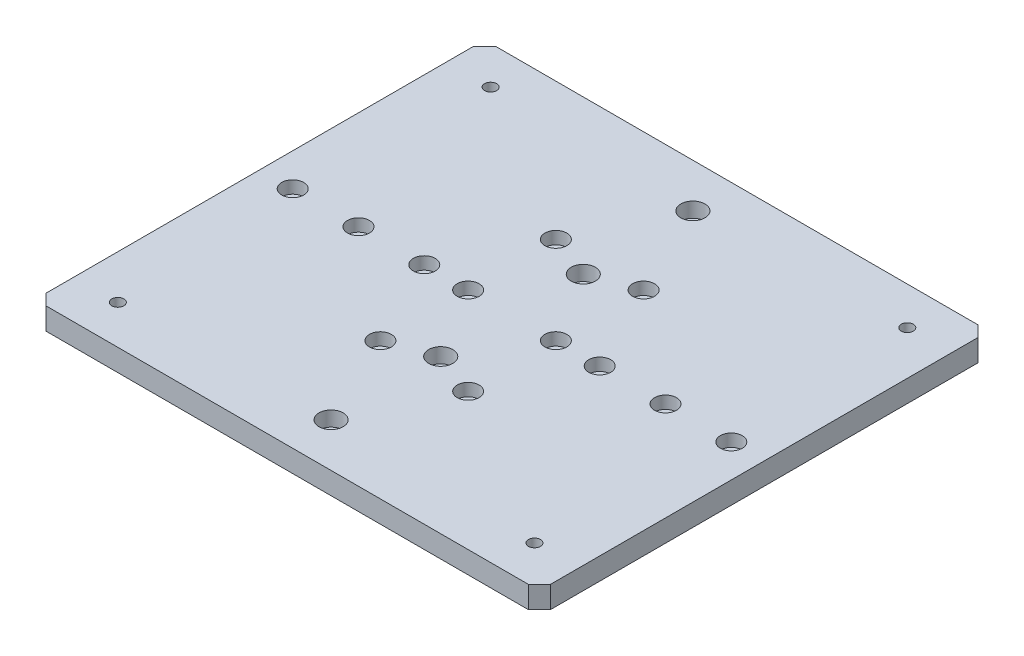
from build123d import *

# Parameters (mm, degrees)
SKETCH_1_W                = 230
SKETCH_1_H                = 205
EXTRUDE_1_DEPTH           = 10
HOLE_WIZARD_1_D           = 5.5
HOLE_WIZARD_1_DEPTH       = 12.4
HOLE_WIZARD_1_CBORE_D     = 10
HOLE_WIZARD_1_CBORE_DEPTH = 5.7
HOLE_WIZARD_1_TIP         = 1.652366702
HOLE_WIZARD_2_D           = 5.5
HOLE_WIZARD_2_DEPTH       = 12.4
HOLE_WIZARD_2_CBORE_D     = 10
HOLE_WIZARD_2_CBORE_DEPTH = 5.7
HOLE_WIZARD_2_TIP         = 1.652366702
CHAMFER_1_SIZE            = 5
HOLE_WIZARD_3_D           = 6.6
HOLE_WIZARD_3_DEPTH       = 12.4
HOLE_WIZARD_3_CBORE_D     = 11
HOLE_WIZARD_3_CBORE_DEPTH = 6.8
HOLE_WIZARD_3_TIP         = 1.982840043


with BuildPart() as part:
    # 草图1 → 凸台-拉伸1 (new body)
    with BuildSketch(Plane(origin=(0, 0, 0), x_dir=(1, 0, 0), z_dir=(0, 1, 0))):
        Rectangle(SKETCH_1_W, SKETCH_1_H)
    extrude(amount=EXTRUDE_1_DEPTH)

    # 打孔尺寸(%根据)内六角圆柱头螺钉的类型1
    with Locations(Plane(origin=(0, 0, 0), x_dir=(-1, 0, 0), z_dir=(0, -1, 0))):
        with Locations((-95, -84.75), (-95, 85.25), (95, -84.75), (95, 85.25)):
            CounterBoreHole(HOLE_WIZARD_1_D / 2, HOLE_WIZARD_1_CBORE_D / 2, HOLE_WIZARD_1_CBORE_DEPTH, depth=HOLE_WIZARD_1_DEPTH)
            with Locations((0, 0, -(HOLE_WIZARD_1_DEPTH + HOLE_WIZARD_1_TIP / 2))):  # 118° drill point
                Cone(0, HOLE_WIZARD_1_D / 2, HOLE_WIZARD_1_TIP, mode=Mode.SUBTRACT)

    # 打孔尺寸(%根据)内六角圆柱头螺钉的类型2
    with Locations(Plane(origin=(0, 10, 0), x_dir=(1, 0, 0), z_dir=(0, 1, 0))):
        with Locations((-100, 0), (-70, 0), (-40, 0), (-20, 0), (-20, 40), (-20, -40), (20, -40), (40, 0), (20, 0), (70, 0), (100, 0), (20, 40)):
            CounterBoreHole(HOLE_WIZARD_2_D / 2, HOLE_WIZARD_2_CBORE_D / 2, HOLE_WIZARD_2_CBORE_DEPTH, depth=HOLE_WIZARD_2_DEPTH)
            with Locations((0, 0, -(HOLE_WIZARD_2_DEPTH + HOLE_WIZARD_2_TIP / 2))):  # 118° drill point
                Cone(0, HOLE_WIZARD_2_D / 2, HOLE_WIZARD_2_TIP, mode=Mode.SUBTRACT)

    # 倒角1
    chamfer_1_edges = [part.edges().sort_by_distance(p)[0] for p in [
        (115, 5, 102.5),
        (-115, 5, 102.5),
        (-115, 5, -102.5),
        (115, 5, -102.5),
    ]]
    chamfer(chamfer_1_edges, length=CHAMFER_1_SIZE)

    # 打孔尺寸(%根据)内六角圆柱头螺钉的类型3
    with Locations(Plane(origin=(0, 10, 0), x_dir=(1, 0, 0), z_dir=(0, 1, 0))):
        with Locations((0, 82.5), (0, 32.5), (0, -32.5), (0, -82.5)):
            CounterBoreHole(HOLE_WIZARD_3_D / 2, HOLE_WIZARD_3_CBORE_D / 2, HOLE_WIZARD_3_CBORE_DEPTH, depth=HOLE_WIZARD_3_DEPTH)
            with Locations((0, 0, -(HOLE_WIZARD_3_DEPTH + HOLE_WIZARD_3_TIP / 2))):  # 118° drill point
                Cone(0, HOLE_WIZARD_3_D / 2, HOLE_WIZARD_3_TIP, mode=Mode.SUBTRACT)


solid = part.part
